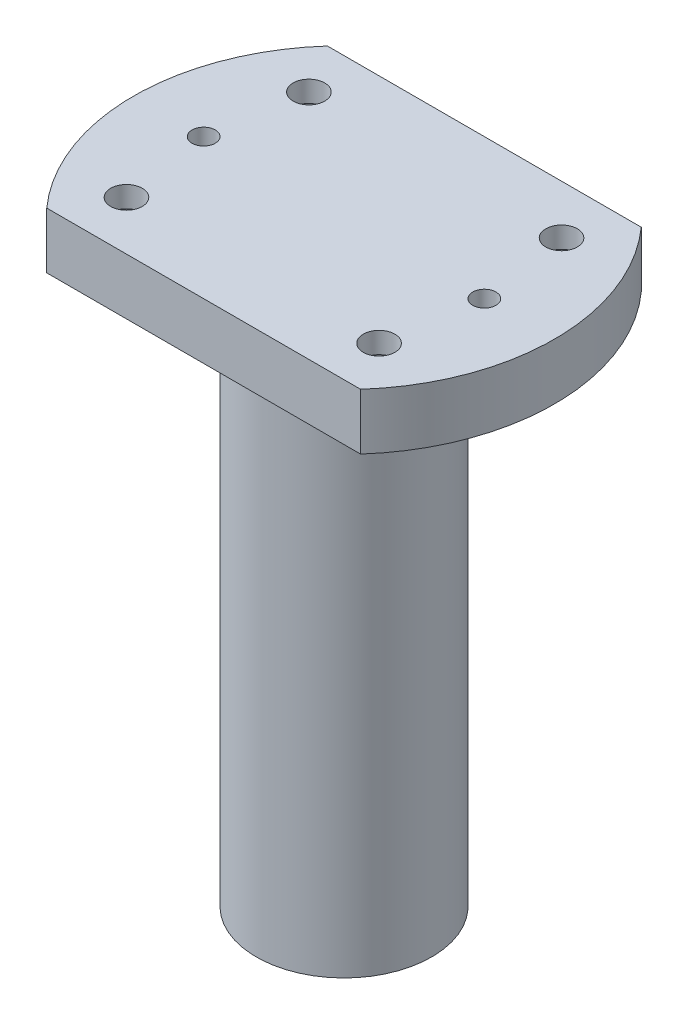
SolidWorks part; units mm, degrees
material "304"
ref_plane "Front Plane" through (0, 0, 0) normal (0, 0, 1) x (1, 0, 0)
ref_plane "Top Plane" through (0, 0, 0) normal (0, 1, 0) x (1, 0, 0)
ref_plane "Right Plane" through (0, 0, 0) normal (1, 0, 0) x (0, 0, -1)
sketch "Sketch1" plane through (0, 0, 0) normal (0, 0, 1) x (1, 0, 0)
  line L0 (0, 0) -> (0, 85) construction
  line L1 (0, 85) -> (-30, 85)
  line L2 (-30, 85) -> (-30, 77)
  line L3 (-30, 77) -> (-12.5, 77)
  line L4 (-12.5, 77) -> (-12.5, 0)
  line L5 (-12.5, 0) -> (0, 0)
  line L6 (0, 0) -> (0, 85)
  dimension "D1" = 8
  dimension "D2" = 85
  dimension "D3" = 12.5
  dimension "D4" = 30
revolve "Revolve1" add sketch "Sketch1" angle 360 about L0
sketch "Sketch2" plane through (0, 0, 0) normal (0, -1, 0) x (-1, 0, 0)
  point P0 (8, 0)
  point P1 (-8, 0)
  dimension "D1" = 16
  dimension "D2" = 8
hole_wizard "M4 Tapped Hole1" positions "3DSketch1" profile "Sketch3" tap size "M4" standard "GB"
sketch3d "3DSketch1"
  point P0 (-8, 0, 0)
  point P3 (8, 0, 0)
sketch "Sketch3" plane through (-8, 0, 0) normal (1, 0, 0) x (0, 0, -1)
  line L0 (0, 0) -> (0, 12.4914)
  line L1 (0, 12.4914) -> (1.65, 11.5)
  line L2 (1.65, 11.5) -> (1.65, 0)
  line L5 (1.65, 0) -> (0, 0)
  line L10 (0, 12.4914) -> (-1.65, 11.5) construction
  line L11 (0, -6.35) -> (0, 107.95) construction
  dimension "螺纹孔钻头直径" = 3.3
  dimension "螺纹孔钻头深度" = 11.5
  dimension "导头角度" = 118
cosmetic thread "Cosmetic Thread3" parameters "D1"=8, "D2"=4
cosmetic thread "Cosmetic Thread4" parameters "D1"=8, "D2"=4
sketch "Sketch4" plane through (0, 85, 0) normal (0, 1, 0) x (1, 0, 0)
  line L0 (33.5323, 0) -> (-37.4689, 0) construction
  line L1 (22.3607, 20) -> (-22.3607, 20)
  line L2 (22.3607, -20) -> (-22.3607, -20)
  line L3 (33.5323, -20) -> (-37.4689, -20) construction
  line L4 (33.5323, 20) -> (-37.4689, 20) construction
  arc A0 (22.3607, 20) -> (-22.3607, 20) centre (0, 0) ccw
  circle A1 centre (0, 0) radius 30
  arc A2 (-22.3607, -20) -> (22.3607, -20) centre (0, 0) ccw
  dimension "D1" = 0
  dimension "D2" = 20
  dimension "D3" = 20
extrude "Cut-Extrude2" cut sketch "Sketch4" against normal up to next
sketch "Sketch5" plane through (0, 77, 0) normal (0, -1, 0) x (1, 0, 0)
  circle A2 centre (20, 0) radius 1.65
  circle A3 centre (-20, 0) radius 1.65
  dimension "D1" = 3.3
  dimension "D2" = 3.3
  dimension "D3" = 20
  dimension "D4" = 40
hole_wizard "CBORE for M4 Hex Head Bolt1" positions "3DSketch2" profile "Sketch6" counterbore size "M4" standard "GB" end condition up to next
sketch3d "3DSketch2"
  point P0 (-20, 77, 0)
  point P3 (20, 77, 0)
sketch "Sketch6" plane through (-20, 77, 0) normal (1, 0, 0) x (0, 0, -1)
  line L0 (0, 0) -> (0, 8)
  line L1 (0, 8) -> (1.5, 8)
  line L3 (1.5, 8) -> (1.5, 3)
  line L4 (1.5, 3) -> (4, 3)
  line L5 (4, 3) -> (4, 0)
  line L7 (4, 0) -> (0, 0)
  line L11 (0, -6.35) -> (0, 107.95) construction
  dimension "通孔孔直径" = 3
  dimension "通孔孔深度" = 8
  dimension "柱形沉头孔直径" = 8
  dimension "柱形沉头孔深度" = 3
hole_wizard "M4 Tapped Hole4" positions "3DSketch5" profile "Sketch9" tap size "M4" standard "GB"
sketch3d "3DSketch5"
  line L0 (20, 85, 0) -> (20, 80, 0) construction
  line L1 (-20, 85, 0) -> (-20, 80, 0) construction
  point P0 (-20, 80, 0)
  point P2 (20, 80, 0)
sketch "Sketch9" plane through (-20, 80, 0) normal (1, 0, 0) x (0, 0, -1)
  line L0 (0, 0) -> (0, 11.0914)
  line L1 (0, 11.0914) -> (1.65, 10.1)
  line L2 (1.65, 10.1) -> (1.65, 0)
  line L5 (1.65, 0) -> (0, 0)
  line L10 (0, 11.0914) -> (-1.65, 10.1) construction
  line L11 (0, -6.35) -> (0, 107.95) construction
  dimension "螺纹孔钻头直径" = 3.3
  dimension "螺纹孔钻头深度" = 10.1
  dimension "导头角度" = 118
cosmetic thread "Cosmetic Thread5" parameters "D1"=8, "D2"=4
cosmetic thread "Cosmetic Thread6" parameters "D1"=8, "D2"=4
sketch "Sketch10" plane through (0, 77, 0) normal (0, -1, 0) x (1, 0, 0)
  line L0 (0, 0) -> (0, 27.8138) construction
  line L1 (0, 0) -> (-49.5574, 0) construction
  circle A0 centre (-18, 13) radius 1.6
  circle A2 centre (-18, -13) radius 1.6
  circle A3 centre (18, -13) radius 1.6
  circle A4 centre (18, 13) radius 1.6
  dimension "D1" = 3.2
  dimension "D2" = 18
  dimension "D3" = 13
hole_wizard "CBORE for M4 Hex Head Bolt2" positions "3DSketch6" profile "Sketch11" counterbore size "M4" standard "GB"
sketch3d "3DSketch6"
  point P0 (-18, 77, 13)
  point P3 (18, 77, 13)
  point P6 (18, 77, -13)
  point P9 (-18, 77, -13)
sketch "Sketch11" plane through (-18, 77, 13) normal (1, 0, 0) x (0, 0, -1)
  line L0 (0, 0) -> (0, 11.4519)
  line L1 (0, 11.4519) -> (2.25, 10.1)
  line L2 (2.25, 10.1) -> (2.25, 5)
  line L3 (2.25, 5) -> (4, 5)
  line L4 (4, 5) -> (4, 0)
  line L5 (4, 0) -> (0, 0)
  line L10 (0, 11.4519) -> (-2.25, 10.1) construction
  line L11 (0, -6.35) -> (0, 107.95) construction
  dimension "孔直径" = 4.5
  dimension "孔深度" = 10.1
  dimension "柱形沉头孔直径" = 8
  dimension "柱形沉头孔深度" = 5
  dimension "导头角度" = 118
